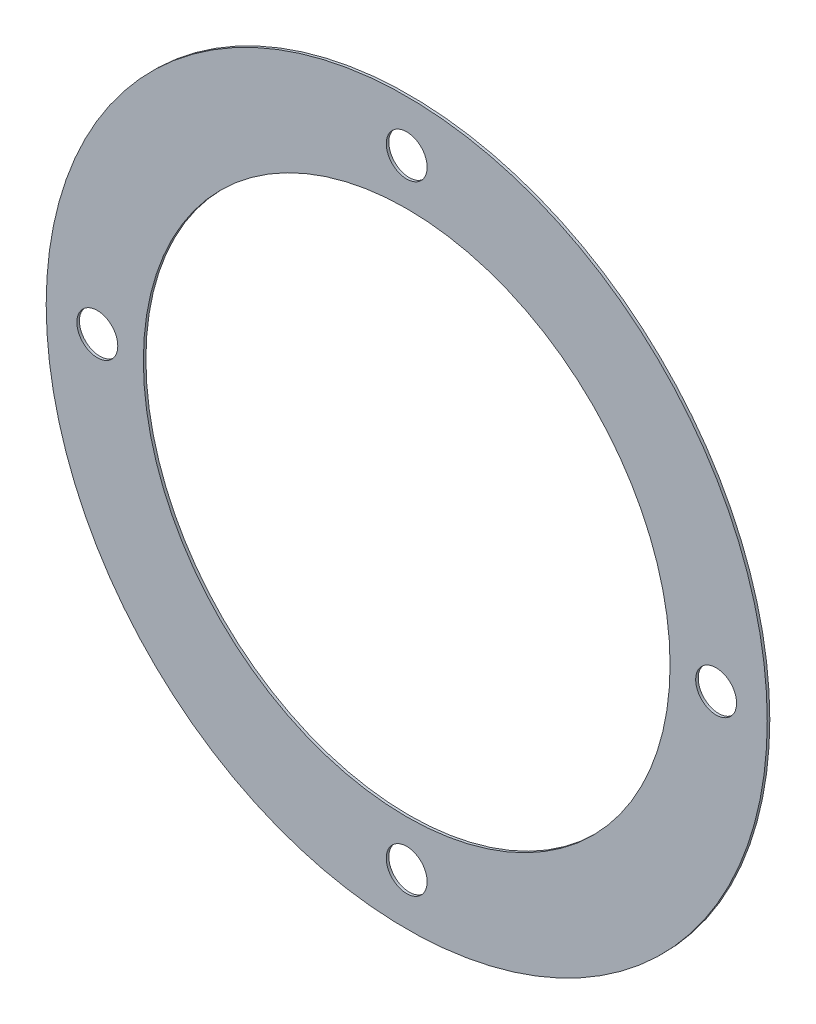
from build123d import *

# Parameters (mm, degrees)
SKETCH1_R           = 70.5
SKETCH1_R_2         = 51.5
BOSS_EXTRUDE1_DEPTH = 0.5
SKETCH2_R           = 4
CUT_EXTRUDE1_DEPTH  = 0.5


with BuildPart() as part:
    # Sketch1 → Boss-Extrude1 (new body)
    with BuildSketch(Plane.XY):
        Circle(SKETCH1_R)
        Circle(SKETCH1_R_2, mode=Mode.SUBTRACT)
    extrude(amount=BOSS_EXTRUDE1_DEPTH)

    # Sketch2 → Cut-Extrude1 (cut)
    with BuildSketch(Plane.XY.offset(0.5)):
        with Locations((0, -60.5)):
            Circle(SKETCH2_R)
        with Locations((-60.5, 0)):
            Circle(SKETCH2_R)
        with Locations((0, 60.5)):
            Circle(SKETCH2_R)
        with Locations((60.5, 0)):
            Circle(SKETCH2_R)
    extrude(amount=-CUT_EXTRUDE1_DEPTH, mode=Mode.SUBTRACT)


solid = part.part
